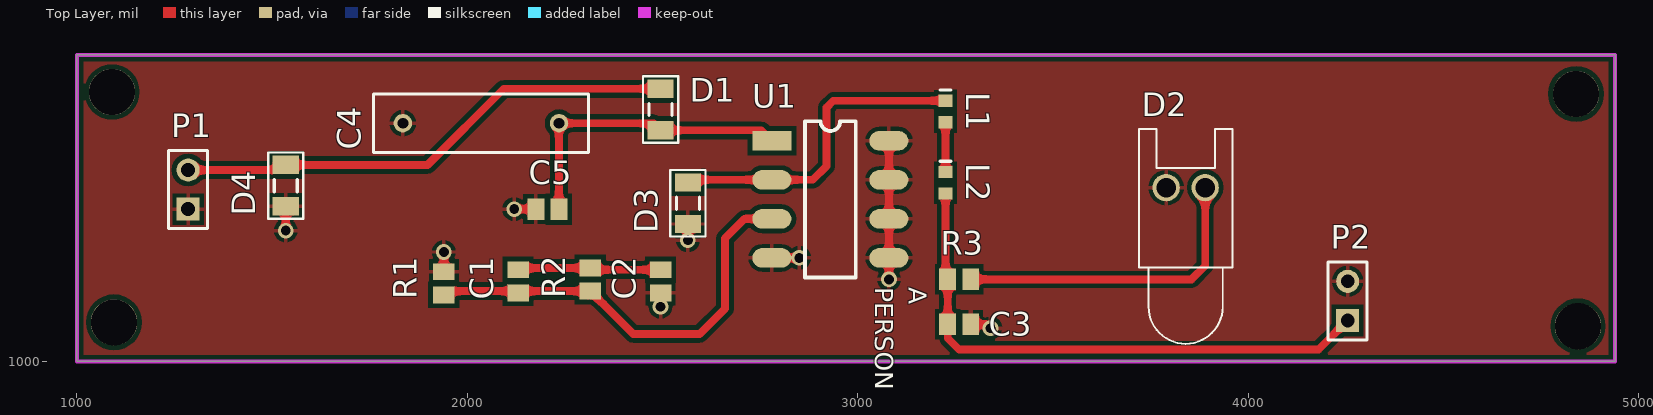
[diagram p0: Top Layer view]
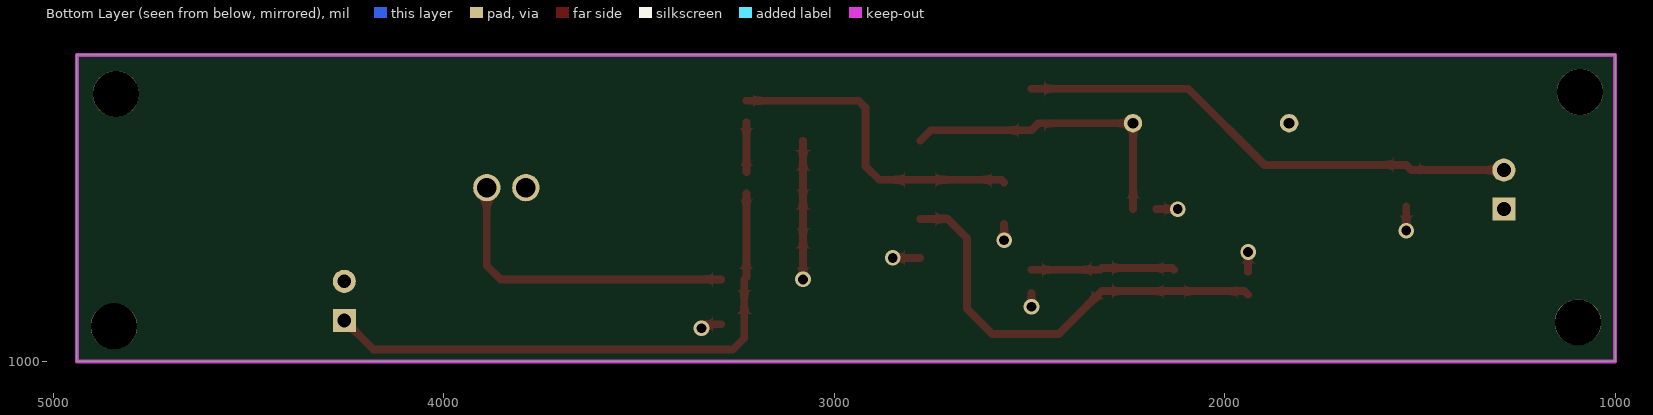
[diagram p1: Bottom Layer view, seen from below]
# Altium PCB MISC84315.PcbDoc
Units mil, origin at the board's own origin, x right, y up, seen from the top; angles counter-clockwise.
Board outline 3940 x 785 mil, 2 copper layers (Top Layer, Bottom Layer); 17 components, 9 nets, 44 pads, 8 vias.

## Layer stack, top to bottom (the 12.6 mil dielectric is the usual default, probably not edited)
Top Solder: solder mask 0.4, Solder Resist, Dk 3.5
Top Layer: signal copper 1.4
Dielectric 1: dielectric 12.6, FR-4, Dk 4.8
Bottom Layer: signal copper 1.4
Bottom Solder: solder mask 0.4, Solder Resist, Dk 3.5

## Board outline
1000,1000 1000,1785 4940,1785 4940,1000

## Design rules (kind name [scope] priority, off if disabled: settings)
Clearance [All] p1: gap=12
MinimumSolderMaskSliver [All] p1: minsoldermaskwidth=0
PolygonConnect [All] p1: connectstyle=Relief reliefconductorwidth=10 reliefentries=4 polygonreliefangle="90 Angle" airgapwidth=10
RoutingVias [All] p1: holewidth=28 width=50 viastyle="Through Hole" minholewidth=28 minwidth=50 maxholewidth=28 maxwidth=50
SilkToSilkClearance [All] p1: silktosilkclearance=0
SilkToSolderMaskClearance [IsPad] p1: minsilkscreentomaskgap=0 clearancetoexposedcopper=TRUE
SolderMaskExpansion [All] p1: expansion=4
Width [All] p1: maxlimit=39.37 minlimit=10 preferedwidth=10
27 further rules are at their usual default settings.

## Components (designator, comment, footprint, x,y, rotation, side; value= is the part's Value field where it differs from the comment)
C1 "6.6UF" C0805 2130,1205 r90 top
C2 "220UF" C0805 2495,1205 r90 top
C3 "220UF" C0805 3260,1095 r180 top
C4 "220UF" RAD-0.4 2035,1610 r180 top
C5 "1UF" C0805 2205,1390 r0 top
D1 "SS36F" C1206 2495,1645 r270 top
D2 "LED0" LED-0 3840,1445 r0 top
D3 "SS36F" C1206 2565,1405 r90 top
D4 "SMBJ48CA" C1206 1535,1450 r90 top
L1 "68UH" INDC1608L 3225,1640 r270 top
L2 "Inductor" INDC1608L 3225,1457.44 r270 top
P1 "Header 2" HDR1X2 1285,1390 r90 top
P2 "Header 2" HDR1X2 4255,1105 r90 top
R1 "2.2K" C0805 1940,1200 r270 top
R2 "6.8K" C0805 2315,1209.53 r90 top
R3 "Res2" C0805 3260,1210 r0 top
U1 "XL1509" ESOP8 2780,1565 r0 top

## Footprints (in the part's own frame and the unit in brackets; to place one, negate y for a bottom-side part, rotate by r counter-clockwise, add the part's x,y. Pads: shape width x height; smd on the part's side, far side on the other; paste and mask are expansions set on the pad)
C0805 [mm] "Chip Capacitor, Body 2.0x1.3mm, IPC High Density"
  rect 1.1x1.4 smd: 1(-0.75,0) 2(0.75,0)
  body extent -1.1,-0.72 1.1,0.72, height 1.4
C1206 [mm]
  rect 1.2x1.7 smd: 1(-1.35,0) 2(1.35,0)
  silkscreen extent -2.16,-1.14 2.16,1.14, body extent -1.7,-0.9 1.7,0.9, height 1.3
ESOP8 [mil]
  rect 100x50 smd: 1(0,0)
  oval 100x50 smd: 2(0,-100) 3(0,-200) 4(0,-300) 5(300,-300) 6(300,-200) 7(300,-100) 8(300,0)
  silkscreen extent 85,-350 215,50
HDR1X2 [mm] "Connector; Header; 2 Position"
  rect 1.5x1.5 hole 0.9: 1(0,0)
  round 1.5 hole 0.9: 2(2.54,0)
  silkscreen extent -1.27,-1.27 3.81,1.27
INDC1608L [mm] "Chip Inductor, Body 1.6x0.8mm, IPC High Density"
  rect 0.8x0.9 smd: 1(-0.7,0) 2(0.7,0)
  silkscreen extent -1.4,-0.35 -1.4,0.35, body extent -0.87,-0.48 0.87,0.48, height 0.55
LED-0 [mil] "LED; 2 Leads"
  round 70 hole 50: 1(50,0) 2(-50,0)
  silkscreen extent -120,-400 120,150
RAD-0.4 [mm] "Radial Cap, Thru-Hole; 2 Leads; 0.4 in Pin Spacing"
  round 1.2 hole 0.7: 1(-5.08,0) 2(5.08,0)
  silkscreen extent -6.98,-1.91 6.98,1.91

## Part data
C1 C2 C3 C5: library part Cap, "Capacitor"
C4: library part "Cap Pol1", "Polarized Capacitor (Radial)"
D1 D3 D4: library part "D Schottky", "Schottky Diode"
D2: "Typical INFRARED GaAs LED"
L1: library part Inductor, "Inductor"
P1 P2: "Header, 2-Pin"
R1 R2: library part Res2, "Resistor"
R3: "Resistor"

## Free pads (board coordinates)
  round 118.11 hole 118.11: 0(1090,1690) 1(1095,1100) 2(4845,1090) 3(4840,1685)

## Via types
v1: diameter 40, hole 25, Top Layer to Bottom Layer, 8 vias

## Nets (pads, with @x,y where several pads share a name; then routed paths per layer and width w, separated by ;. In a path a pad name is that pad's centre, name@x,y a point inside that pad or via, vN(x,y) a via of type N, cw(c..) or ccw(c..) an arc to the next point about the centre after c; other vN are vias at no path point)
+5V: C3.2 L2.2 P2.1 R3.1 | length 1440.4
  Top Layer w20: L2.2 3225,1215.47 R3.1 C3.2 3230.47,1059.53 3260,1030 4180,1030 P2.1
GND: C2.1 C3.1 C4.2 C5.1 D2.2 D3.1 D4.1 P1.1 P2.2 R1.1 U1.4 U1.5 U1.6 U1.7 U1.8 | length 730.6
  Top Layer w20: v1(1535,1335) D4.1 ; R1.1 v1(1940,1280) ; v1@2110,1390 C5.1 ; v1(2495,1140) C2.1 ; v1(2565,1310) D3.1 ; U1.4 v1(2850,1265) ; v1(3080,1210) U1.5 U1.6 U1.7 U1.8 ; C3.1 v1@3340,1095
  other v1: 3340,1085 2120,1390
NetC1_1: C1.1 R1.2 R2.1 U1.3 | length 1117.1
  Top Layer w20: R1.2 1949.53,1180 R2.1 2425,1070 2595,1070 2660,1135 2660,1315 2710,1365 U1.3
NetC1_2: C1.2 C2.2 R2.2 | length 368.8
  Top Layer w20: C1.2 2134.53,1239.06 R2.2 2319.53,1234.53 C2.2
NetC4_1: C4.1 C5.2 D1.2 U1.1 | length 783.8
  Top Layer w20: C5.2 2234.53,1609.53 C4.1 2476.85,1610 D1.2 2753.15,1591.85 U1.1
NetD2_1: D2.1 R3.2 | length 815
  Top Layer w20: R3.2 3855,1210 3890,1245 D2.1
NetD3_2: D3.2 L1.1 U1.2 | length 834.6
  Top Layer w20: D3.2 2571.85,1465 U1.2 2885,1465 2920,1500 2920,1650 2937.56,1667.56 L1.1
NetL1_2: L1.2 L2.1 | length 127.4
  Top Layer w20: L2.1 L1.2
V+: D1.1 D4.2 P1.2 | length 1296.2
  Top Layer w20: P1.2 1521.85,1490 D4.2 1898.15,1503.15 2093.15,1698.15 D1.1

## Polygon pours and split planes (outlines as drawn)
GND on Top Layer "D" (solid, remove dead copper, pour order 0): 770,1905 795,1930 5315,1930 5315,1090 5005,780 4975,750 725,750

## Keep-outs
Keep-Out Layer:
  lines w10: 1000,1000 1000,1785 1835,1785 4940,1785 4940,1000 1000,1000

## Silkscreen, mask and mechanical layers (free items; w line width, h text height)
Top Overlay: